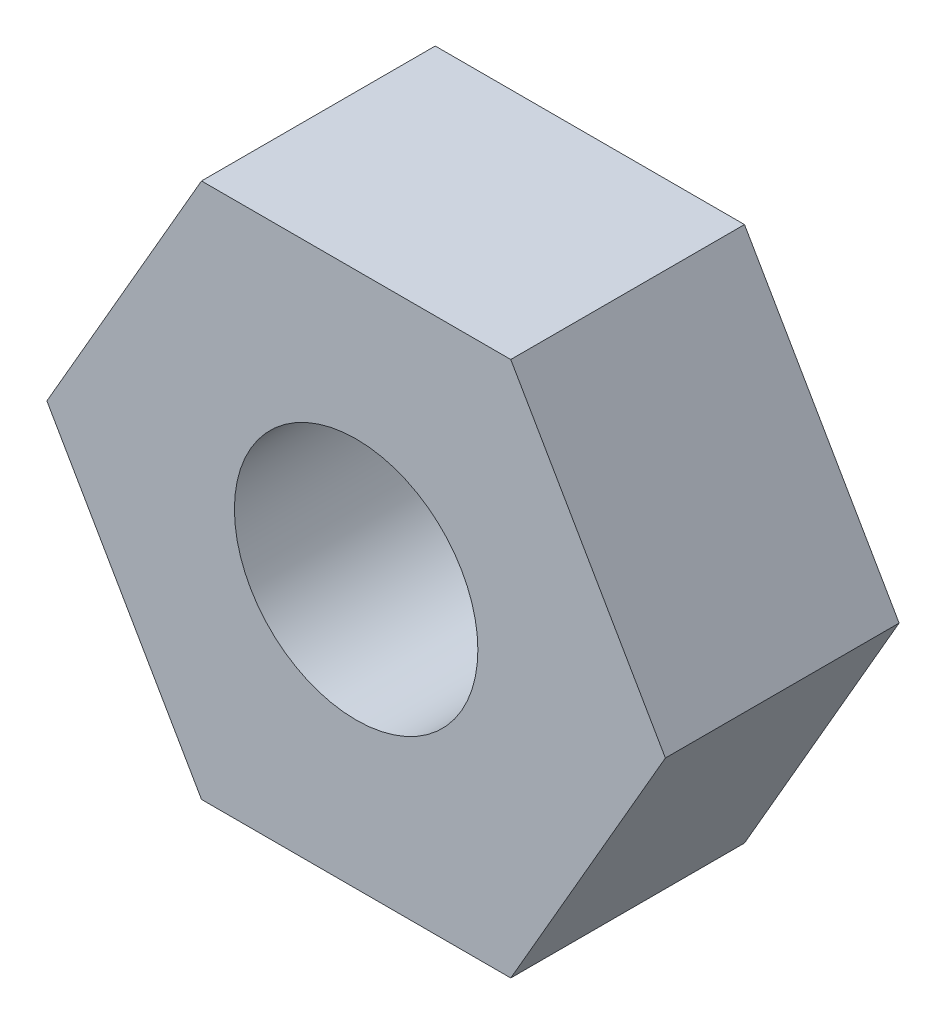
SolidWorks part; units mm, degrees
ref_plane "前视基准面" through (0, 0, 0) normal (0, 0, 1) x (1, 0, 0)
ref_plane "上视基准面" through (0, 0, 0) normal (0, 1, 0) x (1, 0, 0)
ref_plane "右视基准面" through (0, 0, 0) normal (1, 0, 0) x (0, 0, -1)
other "Configuration Table"
sketch "草图1" plane through (0, 0, 0) normal (0, 0, 1) x (1, 0, 0)
  line L0 (3.1754, 0) -> (1.5877, 2.75)
  line L1 (1.5877, 2.75) -> (-1.5877, 2.75)
  line L2 (-1.5877, 2.75) -> (-3.1754, 0)
  line L3 (-3.1754, 0) -> (-1.5877, -2.75)
  line L4 (-1.5877, -2.75) -> (1.5877, -2.75)
  line L5 (1.5877, -2.75) -> (3.1754, 0)
  circle A0 centre (0, 0) radius 1.25
  point P0 (0, 0)
  dimension "D1" = 2.5
  dimension "D2" = 1.5877
  dimension "D3" = 3.1754
  dimension "D4" = 4.7631
  dimension "D5" = 6.3509
  dimension "D6" = 2.75
  dimension "D7" = 5.5
extrude "凸台-拉伸1" add sketch "草图1" against normal mid plane 2.4
